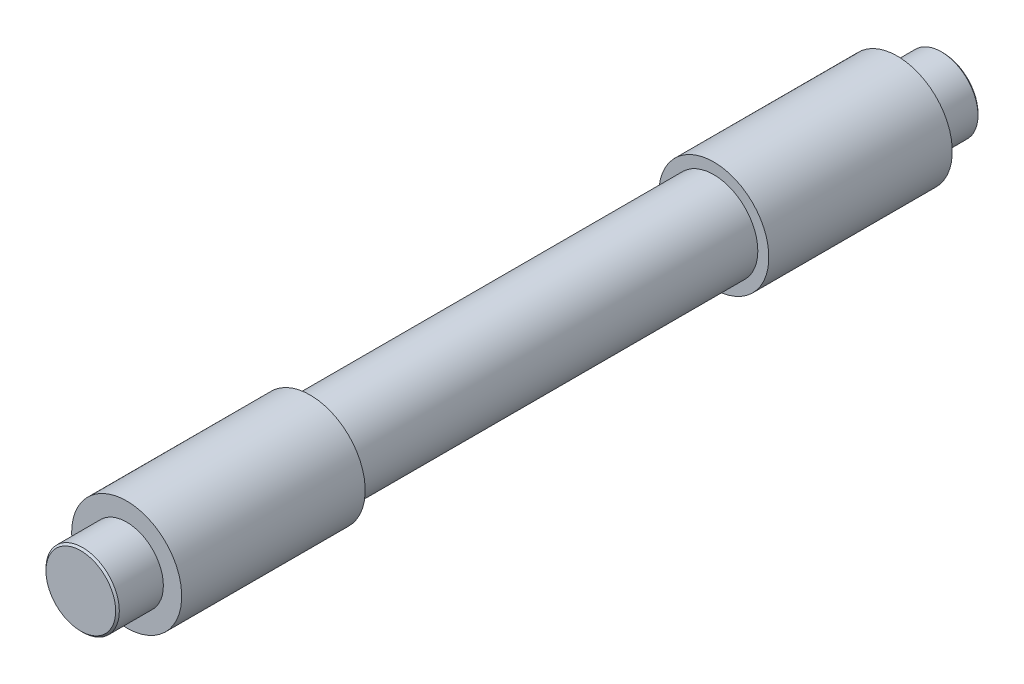
from build123d import *

# Parameters (mm, degrees)
SKETCH_2_R          = 30
EXTRUDE_1_DEPTH     = 470
CUT_EXTRUDE_START   = -25
SKETCH_3_R          = 30
SKETCH_3_R_2        = 20
CUT_EXTRUDE_1_DEPTH = 25
SKETCH_4_R          = 30
SKETCH_4_R_2        = 20
CUT_EXTRUDE_2_DEPTH = 25
SKETCH_5_W          = 6
SKETCH_5_H          = 220


with BuildPart() as part:
    # 草图2 → 凸台-拉伸1 (new body)
    with BuildSketch(Plane.XY):
        with Locations(Location((0, 0, 0), (0, 0, 180))):
            Circle(SKETCH_2_R)
    extrude(amount=EXTRUDE_1_DEPTH)

    # 草图3 → 切除-拉伸1 (cut)
    with BuildSketch(Plane.XY.offset(470).offset(CUT_EXTRUDE_START)):
        with Locations(Location((0, 0, 0), (0, 0, 180))):
            Circle(SKETCH_3_R)
        Circle(SKETCH_3_R_2, mode=Mode.SUBTRACT)
    extrude(amount=CUT_EXTRUDE_1_DEPTH, mode=Mode.SUBTRACT)

    # 草图4 → 切除-拉伸2 (cut)
    with BuildSketch(Plane(origin=(0, 0, 0), x_dir=(-1, 0, 0), z_dir=(0, 0, -1))):
        Circle(SKETCH_4_R)
        with Locations(Location((0, 0, 0), (0, 0, 180))):
            Circle(SKETCH_4_R_2, mode=Mode.SUBTRACT)
    extrude(amount=-CUT_EXTRUDE_2_DEPTH, mode=Mode.SUBTRACT)

    # 草图5 → 切除-旋转1 (revolve, cut)
    with BuildSketch(Plane(origin=(0, 0, 0), x_dir=(1, 0, 0), z_dir=(0, 1, 0))):
        with Locations((-27, -235)):
            Rectangle(SKETCH_5_W, SKETCH_5_H)
    revolve(axis=Axis((0, 0, 345), (0, 0, -1)), mode=Mode.SUBTRACT)

    # 草图6 → 切除-旋转2 (revolve, cut)
    with BuildSketch(Plane(origin=(0, 0, 0), x_dir=(1, 0, 0), z_dir=(0, 1, 0))):
        Polygon((20, -470), (19, -470), (20, -469), align=None)
        Polygon((20, -1), (19, 0), (20, 0), align=None)
    revolve(axis=Axis((0, 0, 470), (0, 0, -1)), mode=Mode.SUBTRACT)


solid = part.part
